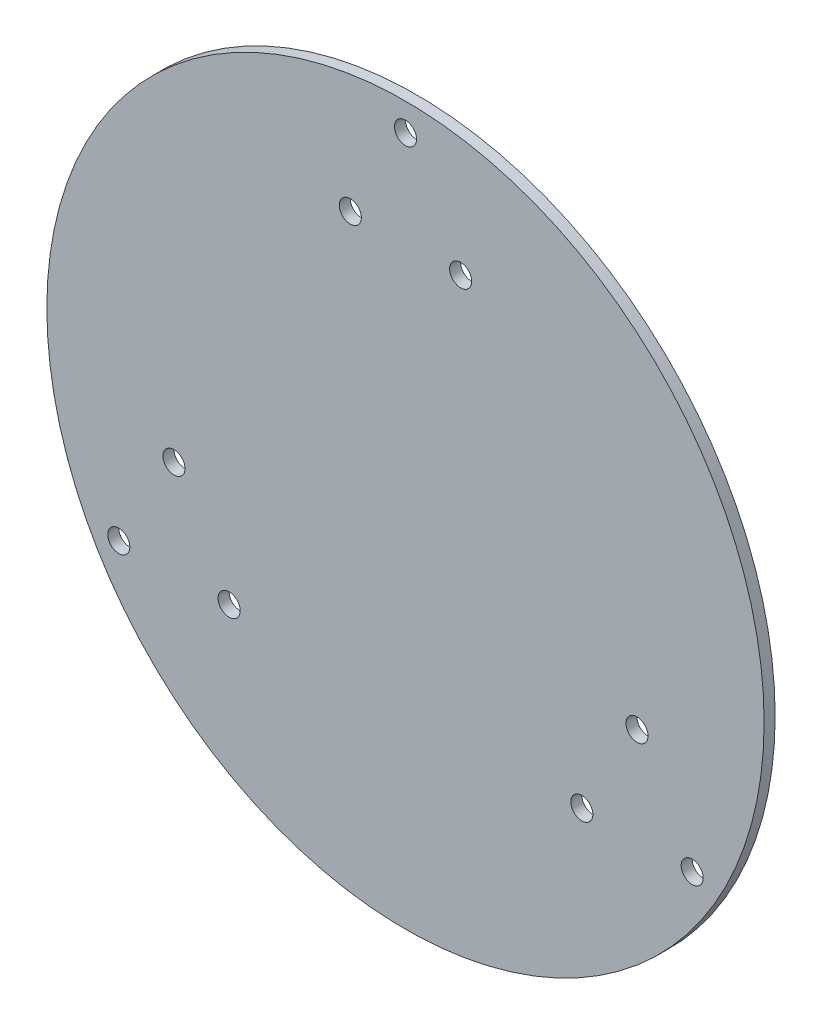
SolidWorks part; units mm, degrees
ref_plane "Front Plane" through (0, 0, 0) normal (0, 0, 1) x (1, 0, 0)
ref_plane "Top Plane" through (0, 0, 0) normal (0, 1, 0) x (1, 0, 0)
ref_plane "Right Plane" through (0, 0, 0) normal (1, 0, 0) x (0, 0, -1)
sketch "Sketch1" plane through (0, 0, 0) normal (0, 0, 1) x (1, 0, 0)
  circle A0 centre (0, 0) radius 65
extrude "Boss-Extrude1" add sketch "Sketch1" along normal blind 2
sketch "Sketch2" plane through (0, 0, 2) normal (0, 0, 1) x (1, 0, 0)
  line L0 (0, 79.4933) -> (0, -85.1939) construction
  line L1 (81.7791, 47.2152) -> (-81.7791, -47.2152) construction
  line L2 (-81.7791, 47.2152) -> (81.7791, -47.2152) construction
  point P6 (0, 0)
  dimension "D1" = 120
sketch "Sketch3" plane through (0, 0, 2) normal (0, 0, 1) x (1, 0, 0)
  line L0 (0, 79.4933) -> (0, -85.1939) construction
  line L1 (0, 60) -> (-10, 42.6795) construction
  line L2 (-10, 42.6795) -> (10, 42.6795) construction
  line L3 (10, 42.6795) -> (0, 60) construction
  circle A0 centre (0, 60) radius 2
  circle A1 centre (10, 42.6795) radius 2
  circle A2 centre (-10, 42.6795) radius 2
  circle A3 centre (31.9615, -30) radius 2
  circle A4 centre (41.9615, -12.6795) radius 2
  circle A5 centre (51.9615, -30) radius 2
  circle A6 centre (-41.9615, -12.6795) radius 2
  circle A7 centre (-31.9615, -30) radius 2
  circle A8 centre (-51.9615, -30) radius 2
  point P24 (0, 0)
  dimension "D1" = 60
  dimension "D5" = 4
  dimension "D6" = 4
  dimension "D7" = 4
  dimension "D2" = 20
  dimension "D3" = 20
  dimension "D4" = 20
  dimension "D8" = 3
extrude "Cut-Extrude1" cut sketch "Sketch3" against normal through all
